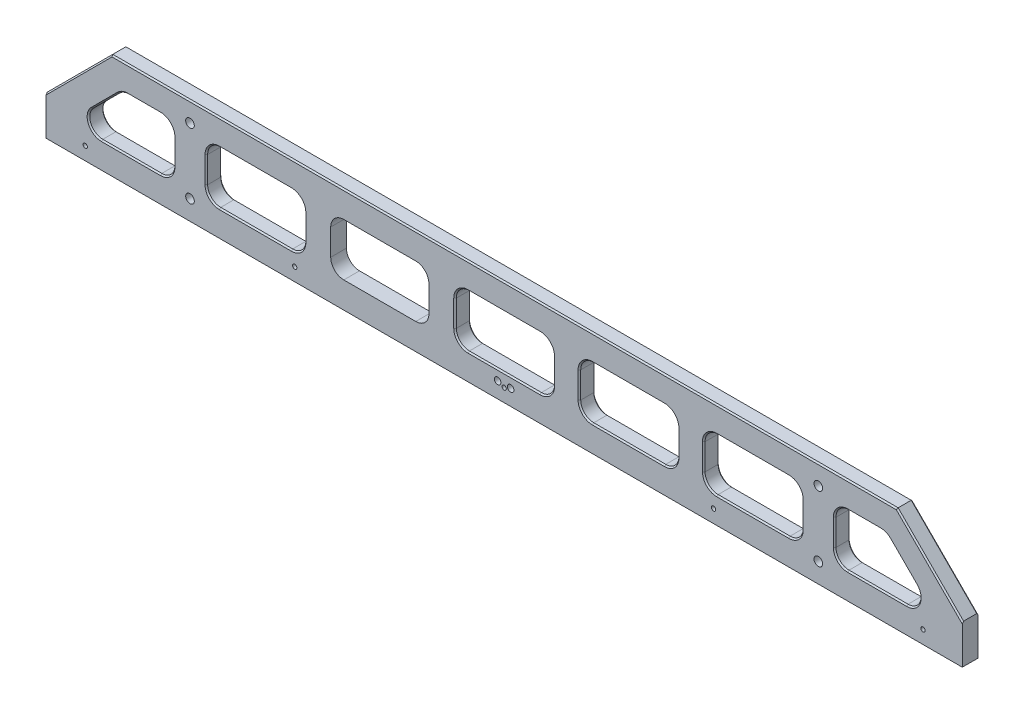
from build123d import *

# Parameters (mm, degrees)
EXTRUDE_1_DEPTH              = 12
SKETCH_2_W                   = 75
SKETCH_2_H                   = 40
CUT_EXTRUDE_1_DEPTH          = 354.393221082
CUT_EXTRUDE_2_DEPTH          = 354.393221082
SKETCH_4_W                   = 75
SKETCH_4_H                   = 40
CUT_EXTRUDE_3_DEPTH          = 354.393221082
SKETCH_5_W                   = 75
SKETCH_5_H                   = 40
CUT_EXTRUDE_4_DEPTH          = 354.393221082
SKETCH_6_W                   = 75
SKETCH_6_H                   = 40
CUT_EXTRUDE_5_DEPTH          = 354.393221082
CUT_EXTRUDE_6_DEPTH          = 354.393221082
SKETCH_8_W                   = 75
SKETCH_8_H                   = 40
CUT_EXTRUDE_7_DEPTH          = 354.393221082
HOLE_WIZARD_3_3_3_3_1_D      = 3.3
HOLE_WIZARD_5_0_5_1_D        = 5
HOLE_WIZARD_M6_1_D           = 6.6
HOLE_WIZARD_M6_1_CBORE_D     = 11
HOLE_WIZARD_M6_1_CBORE_DEPTH = 6.4
HOLE_WIZARD_5_0_5_2_D        = 5
HOLE_WIZARD_5_0_5_2_DEPTH    = 15
HOLE_WIZARD_5_0_5_2_TIP      = 1.502151548
FILLET_1_R                   = 10
CHAMFER_1_SIZE               = 1


with BuildPart() as part:
    # 草图1 → 凸台-拉伸1 (new body)
    with BuildSketch(Plane(origin=(0, 0, 0), x_dir=(-1, 0, 0), z_dir=(0, 0, -1))):
        Polygon((-300, 32.642120962), (-350, -17.357879038), (-350, -47.357879038), (350, -47.357879038), (350, -17.357879038), (300, 32.642120962), align=None)
    extrude(amount=-EXTRUDE_1_DEPTH)

    # 草图2 → 切除-拉伸1 (cut, through all)
    with BuildSketch(Plane(origin=(0, 0, 0), x_dir=(-1, 0, 0), z_dir=(0, 0, -1))):
        with Locations((95, -7.357879038)):
            Rectangle(SKETCH_2_W, SKETCH_2_H)
    extrude(amount=-CUT_EXTRUDE_1_DEPTH, mode=Mode.SUBTRACT)

    # 草图3 → 切除-拉伸2 (cut, through all)
    with BuildSketch(Plane(origin=(0, 0, 0), x_dir=(-1, 0, 0), z_dir=(0, 0, -1))):
        with BuildLine():
            Line((-291.715728753, 12.642120962), (-314.644660941, -10.286811226))
            ThreePointArc((-314.644660941, -10.286811226), (-316.812388454, -21.184713361), (-307.573593129, -27.357879038))
            Line((-307.573593129, -27.357879038), (-252.5, -27.357879038))
            Line((-252.5, -27.357879038), (-252.5, 12.642120962))
            Line((-252.5, 12.642120962), (-291.715728753, 12.642120962))
        make_face()
    extrude(amount=-CUT_EXTRUDE_2_DEPTH, mode=Mode.SUBTRACT)

    # 草图4 → 切除-拉伸3 (cut, through all)
    with BuildSketch(Plane(origin=(0, 0, 0), x_dir=(-1, 0, 0), z_dir=(0, 0, -1))):
        with Locations((0, -7.357879038)):
            Rectangle(SKETCH_4_W, SKETCH_4_H)
    extrude(amount=-CUT_EXTRUDE_3_DEPTH, mode=Mode.SUBTRACT)

    # 草图5 → 切除-拉伸4 (cut, through all)
    with BuildSketch(Plane(origin=(0, 0, 0), x_dir=(-1, 0, 0), z_dir=(0, 0, -1))):
        with Locations((-190, -7.357879038)):
            Rectangle(SKETCH_5_W, SKETCH_5_H)
    extrude(amount=-CUT_EXTRUDE_4_DEPTH, mode=Mode.SUBTRACT)

    # 草图6 → 切除-拉伸5 (cut, through all)
    with BuildSketch(Plane(origin=(0, 0, 0), x_dir=(-1, 0, 0), z_dir=(0, 0, -1))):
        with Locations((190, -7.357879038)):
            Rectangle(SKETCH_6_W, SKETCH_6_H)
    extrude(amount=-CUT_EXTRUDE_5_DEPTH, mode=Mode.SUBTRACT)

    # 草图7 → 切除-拉伸6 (cut, through all)
    with BuildSketch(Plane(origin=(0, 0, 0), x_dir=(-1, 0, 0), z_dir=(0, 0, -1))):
        with BuildLine():
            Line((291.715728753, 12.642120962), (252.5, 12.642120962))
            Line((252.5, 12.642120962), (252.5, -27.357879038))
            Line((252.5, -27.357879038), (307.573593129, -27.357879038))
            ThreePointArc((307.573593129, -27.357879038), (316.812388454, -21.184713361), (314.644660941, -10.286811226))
            Line((314.644660941, -10.286811226), (291.715728753, 12.642120962))
        make_face()
    extrude(amount=-CUT_EXTRUDE_6_DEPTH, mode=Mode.SUBTRACT)

    # 草图8 → 切除-拉伸7 (cut, through all)
    with BuildSketch(Plane.XY.offset(12)):
        with Locations((95, -7.357879038)):
            Rectangle(SKETCH_8_W, SKETCH_8_H)
    extrude(amount=-CUT_EXTRUDE_7_DEPTH, mode=Mode.SUBTRACT)

    # Ø3.3 (3.3) 直径孔1 (through all)
    with Locations(Plane(origin=(0, 0, 0), x_dir=(-1, 0, 0), z_dir=(0, 0, -1))):
        with Locations((-320, -37.357879038), (-160, -37.357879038), (0, -37.357879038), (160, -37.357879038), (320, -37.357879038)):
            Hole(HOLE_WIZARD_3_3_3_3_1_D / 2)

    # Ø5.0 (5) 直径孔1 (through all)
    with Locations(Plane.XY.offset(12)):
        with Locations((5, -35.357879038), (-5, -35.357879038)):
            Hole(HOLE_WIZARD_5_0_5_1_D / 2)

    # M6 六角头螺栓的柱形沉头孔1 (through all)
    with Locations(Plane(origin=(0, 0, 0), x_dir=(-1, 0, 0), z_dir=(0, 0, -1))):
        with Locations((-240, 17.642120962), (-240, -32.357879038), (240, -32.357879038), (240, 17.642120962)):
            CounterBoreHole(HOLE_WIZARD_M6_1_D / 2, HOLE_WIZARD_M6_1_CBORE_D / 2, HOLE_WIZARD_M6_1_CBORE_DEPTH)

    # Ø5.0 (5) 直径孔2
    with Locations(Plane(origin=(0, -47.357879038, 0), x_dir=(-1, 0, 0), z_dir=(0, -1, 0))):
        with Locations((290, -6), (174, -6), (58, -6), (-58, -6), (-290, -6), (-174, -6)):
            Hole(HOLE_WIZARD_5_0_5_2_D / 2, depth=HOLE_WIZARD_5_0_5_2_DEPTH)
            with Locations((0, 0, -(HOLE_WIZARD_5_0_5_2_DEPTH + HOLE_WIZARD_5_0_5_2_TIP / 2))):  # 118° drill point
                Cone(0, HOLE_WIZARD_5_0_5_2_D / 2, HOLE_WIZARD_5_0_5_2_TIP, mode=Mode.SUBTRACT)

    # 圆角1
    fillet_1_edges = [part.edges().sort_by_distance(p)[0] for p in [
        (-291.715728753, 12.642120962, 6),
        (-252.5, -27.357879038, 6),
        (-252.5, 12.642120962, 6),
        (132.5, -27.357879038, 6),
        (57.5, -27.357879038, 6),
        (57.5, 12.642120962, 6),
        (132.5, 12.642120962, 6),
        (-132.5, -27.357879038, 6),
        (-57.5, -27.357879038, 6),
        (-57.5, 12.642120962, 6),
        (-132.5, 12.642120962, 6),
        (291.715728753, 12.642120962, 6),
        (252.5, 12.642120962, 6),
        (252.5, -27.357879038, 6),
        (-37.5, 12.642120962, 6),
        (-37.5, -27.357879038, 6),
        (37.5, -27.357879038, 6),
        (37.5, 12.642120962, 6),
        (227.5, 12.642120962, 6),
        (152.5, 12.642120962, 6),
        (152.5, -27.357879038, 6),
        (227.5, -27.357879038, 6),
        (-227.5, -27.357879038, 6),
        (-152.5, -27.357879038, 6),
        (-152.5, 12.642120962, 6),
        (-227.5, 12.642120962, 6),
    ]]
    fillet(fillet_1_edges, radius=FILLET_1_R)

    # 倒角1
    chamfer_1_edges = [part.edges().sort_by_distance(p)[0] for p in [
        (-190, -27.357879038, 12),
        (-224.571067812, -24.428946849, 12),
        (-155.428932188, -24.428946849, 12),
        (-227.5, -7.357879038, 12),
        (-152.5, -7.357879038, 12),
        (-224.571067812, 9.713188774, 12),
        (-155.428932188, 9.713188774, 12),
        (-190, 12.642120962, 12),
        (95, 12.642120962, 0),
        (60.428932188, 9.713188774, 0),
        (129.571067812, 9.713188774, 0),
        (57.5, -7.357879038, 0),
        (132.5, -7.357879038, 0),
        (60.428932188, -24.428946849, 0),
        (129.571067812, -24.428946849, 0),
        (95, -27.357879038, 0),
        (316.812388454, -21.184713361, 0),
        (304.644660941, -0.286811226, 0),
        (285.036796564, -27.357879038, 0),
        (291.400427452, 11.880916288, 0),
        (255.428932188, -24.428946849, 0),
        (275.036796564, 12.642120962, 0),
        (252.5, -7.357879038, 0),
        (255.428932188, 9.713188774, 0),
        (37.5, -7.357879038, 0),
        (34.571067812, -24.428946849, 0),
        (34.571067812, 9.713188774, 0),
        (0, -27.357879038, 0),
        (0, 12.642120962, 0),
        (-34.571067812, -24.428946849, 0),
        (-34.571067812, 9.713188774, 0),
        (-37.5, -7.357879038, 0),
        (37.5, -7.357879038, 12),
        (34.571067812, -24.428946849, 12),
        (34.571067812, 9.713188774, 12),
        (0, -27.357879038, 12),
        (0, 12.642120962, 12),
        (-34.571067812, -24.428946849, 12),
        (-34.571067812, 9.713188774, 12),
        (-37.5, -7.357879038, 12),
        (-316.812388454, -21.184713361, 12),
        (-304.644660941, -0.286811226, 12),
        (-285.036796564, -27.357879038, 12),
        (-291.400427452, 11.880916288, 12),
        (-255.428932188, -24.428946849, 12),
        (-275.036796564, 12.642120962, 12),
        (-252.5, -7.357879038, 12),
        (-255.428932188, 9.713188774, 12),
        (224.571067812, -24.428946849, 0),
        (227.5, -7.357879038, 0),
        (190, -27.357879038, 0),
        (224.571067812, 9.713188774, 0),
        (155.428932188, -24.428946849, 0),
        (190, 12.642120962, 0),
        (152.5, -7.357879038, 0),
        (155.428932188, 9.713188774, 0),
        (-224.571067812, 9.713188774, 0),
        (-227.5, -7.357879038, 0),
        (-190, 12.642120962, 0),
        (-224.571067812, -24.428946849, 0),
        (-155.428932188, 9.713188774, 0),
        (-190, -27.357879038, 0),
        (-152.5, -7.357879038, 0),
        (-155.428932188, -24.428946849, 0),
        (255.428932188, 9.713188774, 12),
        (275.036796564, 12.642120962, 12),
        (252.5, -7.357879038, 12),
        (291.400427452, 11.880916288, 12),
        (255.428932188, -24.428946849, 12),
        (304.644660941, -0.286811226, 12),
        (285.036796564, -27.357879038, 12),
        (316.812388454, -21.184713361, 12),
        (-252.5, -7.357879038, 0),
        (-255.428932188, 9.713188774, 0),
        (-255.428932188, -24.428946849, 0),
        (-275.036796564, 12.642120962, 0),
        (-285.036796564, -27.357879038, 0),
        (-291.400427452, 11.880916288, 0),
        (-316.812388454, -21.184713361, 0),
        (-304.644660941, -0.286811226, 0),
        (-325, 7.642120962, 12),
        (325, 7.642120962, 12),
        (0, 32.642120962, 12),
        (325, 7.642120962, 0),
        (0, 32.642120962, 0),
        (-325, 7.642120962, 0),
        (224.571067812, 9.713188774, 12),
        (227.5, -7.357879038, 12),
        (190, 12.642120962, 12),
        (224.571067812, -24.428946849, 12),
        (155.428932188, 9.713188774, 12),
        (190, -27.357879038, 12),
        (152.5, -7.357879038, 12),
        (155.428932188, -24.428946849, 12),
        (95, 12.642120962, 12),
        (129.571067812, 9.713188774, 12),
        (60.428932188, 9.713188774, 12),
        (132.5, -7.357879038, 12),
        (57.5, -7.357879038, 12),
        (129.571067812, -24.428946849, 12),
        (60.428932188, -24.428946849, 12),
        (95, -27.357879038, 12),
    ]]
    chamfer(chamfer_1_edges, length=CHAMFER_1_SIZE)


solid = part.part
